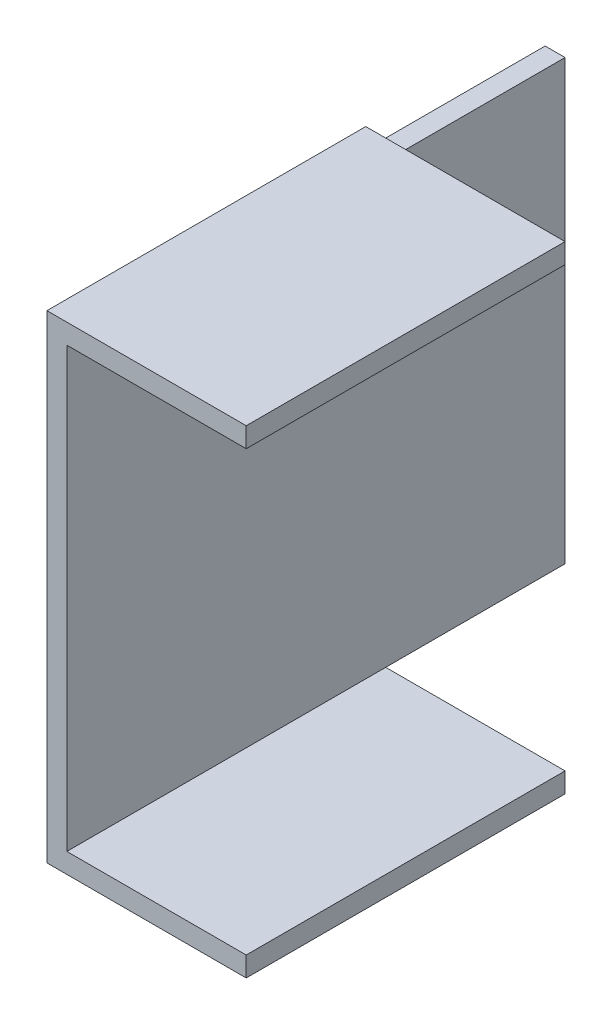
SolidWorks part; units mm, degrees
ref_plane "前视基准面" through (0, 0, 0) normal (0, 0, 1) x (1, 0, 0)
ref_plane "上视基准面" through (0, 0, 0) normal (0, 1, 0) x (1, 0, 0)
ref_plane "右视基准面" through (0, 0, 0) normal (1, 0, 0) x (0, 0, -1)
sketch "草图1" plane through (0, 0, 0) normal (0, 0, 1) x (1, 0, 0)
  line L0 (0, 0) -> (0, 120)
  line L1 (0, 120) -> (50, 120)
  line L2 (0, 0) -> (50, 0)
  line L3 (5, 5) -> (50, 5)
  line L4 (5, 5) -> (5, 115)
  line L5 (5, 115) -> (50, 115)
  line L6 (50, 115) -> (50, 120)
  line L7 (50, 0) -> (50, 5)
  dimension "D1" = 5
extrude "凸台-拉伸1" add sketch "草图1" against normal blind 150
sketch "草图2" plane through (0, 0, -150) normal (0, 0, -1) x (-1, 0, 0)
  line L0 (-50, 120) -> (0, 120)
  line L1 (0, 120) -> (0, 115)
  line L2 (0, 120) -> (0, 0) construction
  line L3 (0, 115) -> (-50, 115)
  line L4 (-50, 115) -> (-50, 120)
  line L5 (-50, 5) -> (0, 5)
  line L6 (0, 5) -> (0, 0)
  line L7 (0, 0) -> (-50, 0)
  line L8 (-50, 0) -> (-50, 5)
extrude "切除-拉伸1" cut sketch "草图2" against normal blind 45
sketch "草图3" plane through (0, 0, -150) normal (0, 0, -1) x (-1, 0, 0)
  line L8 (-5, 115) -> (-5, 5)
  line L9 (-5, 5) -> (0, 5)
  line L10 (0, 5) -> (0, 115)
  line L11 (0, 115) -> (-5, 115)
  line L12 (-5, 115) -> (-5, 5)
  line L13 (-5, 5) -> (0, 5)
  line L14 (0, 5) -> (0, 115)
  line L15 (0, 115) -> (-5, 115)
  dimension "D1" = 0
extrude "切除-拉伸2" cut sketch "草图3" against normal blind 25
sketch "草图4" plane through (0, 0, -105) normal (0, 0, -1) x (-1, 0, 0)
  line L10 (-50, 120) -> (-50, 115)
  line L11 (-50, 115) -> (-5, 115)
  line L12 (-5, 115) -> (0, 115)
  line L13 (0, 115) -> (0, 120)
  line L14 (0, 120) -> (-50, 120)
  line L15 (-50, 120) -> (-50, 115)
  line L16 (-50, 115) -> (-5, 115)
  line L17 (-5, 115) -> (0, 115)
  line L18 (0, 115) -> (0, 120)
  line L19 (0, 120) -> (-50, 120)
  dimension "D1" = 0
extrude "切除-拉伸3" cut sketch "草图4" against normal blind 25
sketch "草图5" plane through (0, 0, -105) normal (0, 0, -1) x (-1, 0, 0)
  line L10 (-50, 5) -> (-50, 0)
  line L11 (-50, 0) -> (0, 0)
  line L12 (0, 0) -> (0, 5)
  line L13 (0, 5) -> (-5, 5)
  line L14 (-5, 5) -> (-50, 5)
  line L15 (-50, 5) -> (-50, 0)
  line L16 (-50, 0) -> (0, 0)
  line L17 (0, 0) -> (0, 5)
  line L18 (0, 5) -> (-5, 5)
  line L19 (-5, 5) -> (-50, 5)
  dimension "D1" = 0
extrude "切除-拉伸4" cut sketch "草图5" against normal blind 25
